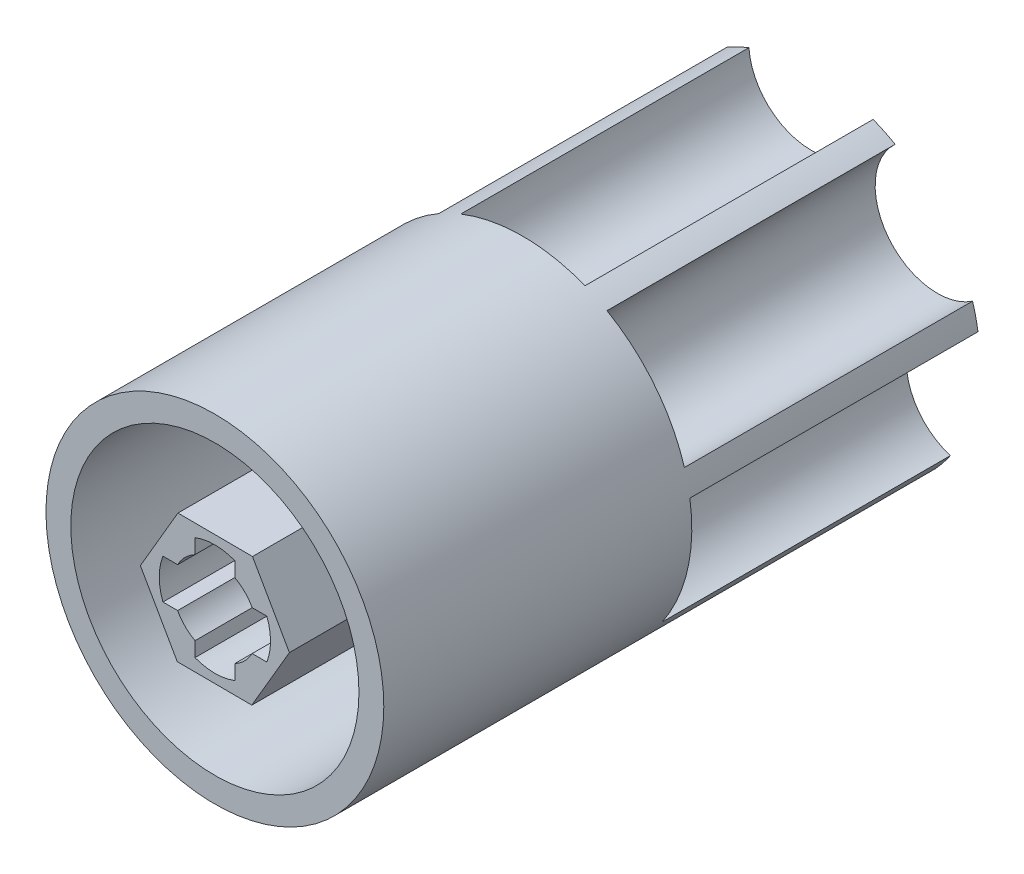
SolidWorks part; units mm, degrees
ref_plane "前视基准面" through (0, 0, 0) normal (0, 0, 1) x (1, 0, 0)
ref_plane "上视基准面" through (0, 0, 0) normal (0, 1, 0) x (1, 0, 0)
ref_plane "右视基准面" through (0, 0, 0) normal (1, 0, 0) x (0, 0, -1)
sketch "草图1" plane through (0, 0, 0) normal (0, 0, 1) x (1, 0, 0)
  line L0 (0, 0) -> (0, 11.2) construction
  line L1 (7.4323, -13.0295) -> (15, -0.0782)
  line L2 (15, -0.0782) -> (7.5677, 12.9513)
  line L3 (7.5677, 12.9513) -> (-7.4323, 13.0295)
  line L4 (-7.4323, 13.0295) -> (-15, 0.0782)
  line L5 (-15, 0.0782) -> (-7.5677, -12.9513)
  line L6 (-7.5677, -12.9513) -> (7.4323, -13.0295)
  line L7 (-4, 10.4614) -> (-4, 7.5)
  line L8 (4, 10.4614) -> (4, 7.5)
  line L9 (10.4614, 4) -> (7.5, 4)
  line L10 (10.4614, -4) -> (7.5, -4)
  line L11 (4, -10.4614) -> (4, -7.5)
  line L12 (-4, -10.4614) -> (-4, -7.5)
  line L13 (-10.4614, -4) -> (-7.5, -4)
  line L14 (-10.4614, 4) -> (-7.5, 4)
  circle A0 centre (0, 0) radius 34
  circle A1 centre (0, 0) radius 29
  circle A2 centre (0, 0) radius 12.9906 construction
  arc A3 (-4, 7.5) -> (-7.5, 4) centre (0, 0) ccw
  arc A4 (4, 10.4614) -> (-4, 10.4614) centre (0, 0) ccw
  arc A5 (7.5, 4) -> (4, 7.5) centre (0, 0) ccw
  circle A6 centre (0, 0) radius 8.5 construction
  circle A7 centre (0, 0) radius 11.2 construction
  arc A8 (10.4614, -4) -> (10.4614, 4) centre (0, 0) ccw
  arc A9 (4, -7.5) -> (7.5, -4) centre (0, 0) ccw
  arc A10 (-4, -10.4614) -> (4, -10.4614) centre (0, 0) ccw
  arc A11 (-7.5, -4) -> (-4, -7.5) centre (0, 0) ccw
  arc A12 (-10.4614, 4) -> (-10.4614, -4) centre (0, 0) ccw
  point P5 (10.7106, 3.2746)
  point P20 (8.1286, 2.4852)
  dimension "D1" = 68
  dimension "D4" = 17
  dimension "D6" = 4
  dimension "D3" = 30
  dimension "D2" = 5
  dimension "D5" = 2.7
  dimension "D7" = 4
extrude "凸台-拉伸1" add sketch "草图1" along normal blind 60 contours A0 A1 | L5 L6 L1 L2 L3 L4 A12 L14 A3 L7 A4 L8 A5 L9 A8 L10 A9 L11 A10 L12 A11 L13
sketch "草图2" plane through (0, 0, 0) normal (0, 0, 1) x (1, 0, 0)
  line L0 (-10.4614, -4) -> (-7.5, -4) construction
  line L1 (-10.4614, 4) -> (-7.5, 4) construction
  line L2 (-4, 10.4614) -> (-4, 7.5) construction
  line L3 (4, 10.4614) -> (4, 7.5) construction
  line L4 (10.4614, 4) -> (7.5, 4) construction
  line L5 (10.4614, -4) -> (7.5, -4) construction
  line L6 (0, 0) -> (0, 34) construction
  line L18 (4, -10.4614) -> (4, -7.5) construction
  line L19 (-4, -10.4614) -> (-4, -7.5) construction
  line L20 (-10.4614, -4) -> (-7.5, -4)
  line L21 (-10.4614, 4) -> (-7.5, 4)
  line L22 (-4, 10.4614) -> (-4, 7.5)
  line L23 (4, 10.4614) -> (4, 7.5)
  line L24 (10.4614, 4) -> (7.5, 4)
  line L25 (10.4614, -4) -> (7.5, -4)
  line L26 (4, -10.4614) -> (4, -7.5)
  line L27 (-4, -10.4614) -> (-4, -7.5)
  arc A0 (-7.5, -4) -> (-4, -7.5) centre (0, 0) ccw construction
  arc A1 (-10.4614, 4) -> (-10.4614, -4) centre (0, 0) ccw construction
  arc A2 (-4, 7.5) -> (-7.5, 4) centre (0, 0) ccw construction
  arc A3 (4, 10.4614) -> (-4, 10.4614) centre (0, 0) ccw construction
  arc A4 (7.5, 4) -> (4, 7.5) centre (0, 0) ccw construction
  arc A5 (10.4614, -4) -> (10.4614, 4) centre (0, 0) ccw construction
  arc A6 (4, -7.5) -> (7.5, -4) centre (0, 0) ccw construction
  arc A7 (-4, -10.4614) -> (4, -10.4614) centre (0, 0) ccw construction
  arc A8 (-7.5, -4) -> (-4, -7.5) centre (0, 0) ccw
  arc A9 (-10.4614, 4) -> (-10.4614, -4) centre (0, 0) ccw
  arc A10 (-4, 7.5) -> (-7.5, 4) centre (0, 0) ccw
  arc A11 (4, 10.4614) -> (-4, 10.4614) centre (0, 0) ccw
  arc A12 (7.5, 4) -> (4, 7.5) centre (0, 0) ccw
  arc A13 (10.4614, -4) -> (10.4614, 4) centre (0, 0) ccw
  arc A14 (4, -7.5) -> (7.5, -4) centre (0, 0) ccw
  arc A15 (-4, -10.4614) -> (4, -10.4614) centre (0, 0) ccw
  circle A16 centre (0, 0) radius 34 construction
  arc A17 (16.927, 29.4869) -> (12.5, 31.6188) centre (0, 0) ccw
  arc A18 (12.5, 31.6188) -> (-12.5, 31.6188) centre (0, 32.5334) cw
  arc A19 (32.5142, 9.9411) -> (16.927, 29.4869) centre (25.4356, 20.2843) cw
  arc A20 (28.0446, -19.2224) -> (33.6076, 5.1507) centre (31.7177, -7.2394) cw
  arc A21 (2.4568, -33.9111) -> (24.981, -23.064) centre (14.1157, -29.3116) cw
  arc A22 (-24.981, -23.064) -> (-2.4568, -33.9111) centre (-14.1157, -29.3116) cw
  arc A23 (-33.6076, 5.1507) -> (-28.0446, -19.2224) centre (-31.7177, -7.2394) cw
  arc A24 (-16.927, 29.4869) -> (-32.5142, 9.9411) centre (-25.4356, 20.2843) cw
  arc A25 (33.6076, 5.1507) -> (32.5142, 9.9411) centre (0, 0) ccw
  arc A26 (24.981, -23.064) -> (28.0446, -19.2224) centre (0, 0) ccw
  arc A27 (-2.4568, -33.9111) -> (2.4568, -33.9111) centre (0, 0) ccw
  arc A28 (-28.0446, -19.2224) -> (-24.981, -23.064) centre (0, 0) ccw
  arc A29 (-32.5142, 9.9411) -> (-33.6076, 5.1507) centre (0, 0) ccw
  arc A30 (-12.5, 31.6188) -> (-16.927, 29.4869) centre (0, 0) ccw
  point P5 (0, 20)
  dimension "D1" = 20
  dimension "D2" = 25
  dimension "D3" = 7
extrude "凸台-拉伸2" add sketch "草图2" against normal blind 60
sketch "草图4" plane through (0, 0, 0) normal (0, 0, 1) x (1, 0, 0)
  circle A0 centre (0, 0) radius 34 construction
  circle A1 centre (0, 0) radius 34
  arc A16 (28.5837, 4.8959) -> (23.6288, -16.8131) centre (31.7177, -7.2394) ccw
  arc A17 (28.5837, 4.8959) -> (27.8773, 7.991) centre (0, 0) ccw
  arc A18 (13.9939, 25.4002) -> (27.8773, 7.991) centre (25.4356, 20.2843) ccw
  arc A19 (13.9939, 25.4002) -> (11.1336, 26.7776) centre (0, 0) ccw
  arc A20 (-11.1336, 26.7776) -> (11.1336, 26.7776) centre (0, 32.5334) ccw
  arc A21 (-11.1336, 26.7776) -> (-13.9939, 25.4002) centre (0, 0) ccw
  arc A22 (-27.8773, 7.991) -> (-13.9939, 25.4002) centre (-25.4356, 20.2843) ccw
  arc A23 (-27.8773, 7.991) -> (-28.5837, 4.8959) centre (0, 0) ccw
  arc A24 (-23.6288, -16.8131) -> (-28.5837, 4.8959) centre (-31.7177, -7.2394) ccw
  arc A25 (-23.6288, -16.8131) -> (-21.6494, -19.2951) centre (0, 0) ccw
  arc A26 (-1.5873, -28.9565) -> (-21.6494, -19.2951) centre (-14.1157, -29.3116) ccw
  arc A27 (-1.5873, -28.9565) -> (1.5873, -28.9565) centre (0, 0) ccw
  arc A28 (21.6494, -19.2951) -> (1.5873, -28.9565) centre (14.1157, -29.3116) ccw
  arc A29 (21.6494, -19.2951) -> (23.6288, -16.8131) centre (0, 0) ccw
  arc A30 (28.5837, 4.8959) -> (23.6288, -16.8131) centre (31.7177, -7.2394) ccw
  arc A31 (28.5837, 4.8959) -> (27.8773, 7.991) centre (0, 0) ccw
  arc A32 (13.9939, 25.4002) -> (27.8773, 7.991) centre (25.4356, 20.2843) ccw
  arc A33 (13.9939, 25.4002) -> (11.1336, 26.7776) centre (0, 0) ccw
  arc A34 (-11.1336, 26.7776) -> (11.1336, 26.7776) centre (0, 32.5334) ccw
  arc A35 (-11.1336, 26.7776) -> (-13.9939, 25.4002) centre (0, 0) ccw
  arc A36 (-27.8773, 7.991) -> (-13.9939, 25.4002) centre (-25.4356, 20.2843) ccw
  arc A37 (-27.8773, 7.991) -> (-28.5837, 4.8959) centre (0, 0) ccw
  arc A38 (-23.6288, -16.8131) -> (-28.5837, 4.8959) centre (-31.7177, -7.2394) ccw
  arc A39 (-23.6288, -16.8131) -> (-21.6494, -19.2951) centre (0, 0) ccw
  arc A40 (-1.5873, -28.9565) -> (-21.6494, -19.2951) centre (-14.1157, -29.3116) ccw
  arc A41 (-1.5873, -28.9565) -> (1.5873, -28.9565) centre (0, 0) ccw
  arc A42 (21.6494, -19.2951) -> (1.5873, -28.9565) centre (14.1157, -29.3116) ccw
  arc A43 (21.6494, -19.2951) -> (23.6288, -16.8131) centre (0, 0) ccw
  dimension "D1" = 0
extrude "凸台-拉伸3" add sketch "草图4" against normal blind 2 contours A1 A43 A42 A41 A40 A39 A38 A37 A36 A35 A34 A33 A32 A31 A30
